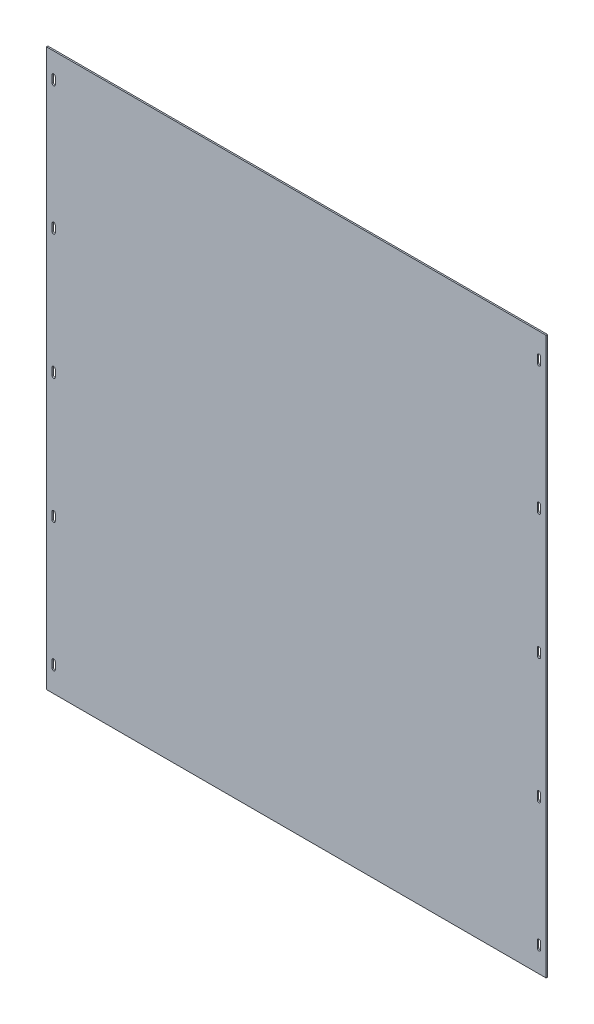
SolidWorks part; units mm, degrees
material "Q235A"
ref_plane "前视基准面" through (0, 0, 0) normal (0, 0, 1) x (1, 0, 0)
ref_plane "上视基准面" through (0, 0, 0) normal (0, 1, 0) x (1, 0, 0)
ref_plane "右视基准面" through (0, 0, 0) normal (1, 0, 0) x (0, 0, -1)
sketch "草图1" plane through (0, 0, 0) normal (0, 0, 1) x (1, 0, 0)
  line L1 (-350, 390) -> (350, 390)
  line L2 (-350, 390) -> (-350, -390)
  line L3 (-350, -390) -> (350, -390)
  line L4 (350, 390) -> (350, -390)
  line L5 (0, -390) -> (0, 390) construction
  line L6 (-350, 0) -> (350, 0) construction
  point P0 (0, 0)
  dimension "D1" = 700
  dimension "D2" = 780
extrude "凸台-拉伸1" add sketch "草图1" along normal blind 2
sketch "草图2" plane through (0, 0, 2) normal (0, 0, 1) x (1, 0, 0)
  line L0 (0, 390) -> (0, -390) construction
  line L1 (350, 390) -> (-350, 390) construction
  line L2 (-350, -390) -> (350, -390) construction
  line L3 (-340, 360) -> (-340, 350) construction
  line L4 (-340, -355) -> (340, -355) construction
  line L5 (-340, -355) -> (-340, 355) construction
  line L6 (-340, 355) -> (340, 355) construction
  line L7 (340, -355) -> (340, 355) construction
  line L8 (0, 355) -> (0, -355) construction
  line L9 (-340, 0) -> (340, 0) construction
  line L10 (-337.75, 360) -> (-337.75, 350)
  line L11 (-342.25, 360) -> (-342.25, 350)
  line L12 (340, 360) -> (340, 350) construction
  line L13 (337.75, 360) -> (337.75, 350)
  line L14 (342.25, 360) -> (342.25, 350)
  line L15 (-340, 170) -> (-340, 180) construction
  line L16 (-342.25, 170) -> (-342.25, 180)
  line L17 (-337.75, 170) -> (-337.75, 180)
  line L18 (-340, -5) -> (-340, 5) construction
  line L19 (-342.25, -5) -> (-342.25, 5)
  line L20 (-337.75, -5) -> (-337.75, 5)
  line L21 (340, 170) -> (340, 180) construction
  line L22 (342.25, 170) -> (342.25, 180)
  line L23 (337.75, 170) -> (337.75, 180)
  line L24 (340, -5) -> (340, 5) construction
  line L25 (342.25, -5) -> (342.25, 5)
  line L26 (337.75, -5) -> (337.75, 5)
  line L27 (-340, 540) -> (-340, 530) construction
  line L28 (-342.25, 540) -> (-342.25, 530)
  line L29 (-337.75, 540) -> (-337.75, 530)
  line L30 (340, 540) -> (340, 530) construction
  line L31 (342.25, 540) -> (342.25, 530)
  line L32 (337.75, 540) -> (337.75, 530)
  line L33 (-340, -355) -> (340, -355) construction
  line L34 (340, -170) -> (340, -180) construction
  line L35 (342.25, -170) -> (342.25, -180)
  line L36 (337.75, -170) -> (337.75, -180)
  line L37 (-340, -170) -> (-340, -180) construction
  line L38 (-342.25, -170) -> (-342.25, -180)
  line L39 (-337.75, -170) -> (-337.75, -180)
  line L40 (340, -360) -> (340, -350) construction
  line L41 (337.75, -360) -> (337.75, -350)
  line L42 (342.25, -360) -> (342.25, -350)
  line L43 (-340, -360) -> (-340, -350) construction
  line L44 (-337.75, -360) -> (-337.75, -350)
  line L45 (-342.25, -360) -> (-342.25, -350)
  arc A0 (-337.75, 360) -> (-342.25, 360) centre (-340, 360) ccw
  arc A1 (-342.25, 350) -> (-337.75, 350) centre (-340, 350) ccw
  arc A2 (337.75, 360) -> (342.25, 360) centre (340, 360) cw
  arc A3 (342.25, 350) -> (337.75, 350) centre (340, 350) cw
  arc A4 (-342.25, 170) -> (-337.75, 170) centre (-340, 170) ccw
  arc A5 (-337.75, 180) -> (-342.25, 180) centre (-340, 180) ccw
  arc A6 (-342.25, -5) -> (-337.75, -5) centre (-340, -5) ccw
  arc A7 (-337.75, 5) -> (-342.25, 5) centre (-340, 5) ccw
  arc A8 (342.25, 170) -> (337.75, 170) centre (340, 170) cw
  arc A9 (337.75, 180) -> (342.25, 180) centre (340, 180) cw
  arc A10 (342.25, -5) -> (337.75, -5) centre (340, -5) cw
  arc A11 (337.75, 5) -> (342.25, 5) centre (340, 5) cw
  arc A12 (-342.25, 540) -> (-337.75, 540) centre (-340, 540) cw
  arc A13 (-337.75, 530) -> (-342.25, 530) centre (-340, 530) cw
  arc A14 (342.25, 540) -> (337.75, 540) centre (340, 540) ccw
  arc A15 (337.75, 530) -> (342.25, 530) centre (340, 530) ccw
  arc A16 (342.25, -170) -> (337.75, -170) centre (340, -170) ccw
  arc A17 (337.75, -180) -> (342.25, -180) centre (340, -180) ccw
  arc A18 (-342.25, -170) -> (-337.75, -170) centre (-340, -170) cw
  arc A19 (-337.75, -180) -> (-342.25, -180) centre (-340, -180) cw
  arc A20 (337.75, -360) -> (342.25, -360) centre (340, -360) ccw
  arc A21 (342.25, -350) -> (337.75, -350) centre (340, -350) ccw
  arc A22 (-337.75, -360) -> (-342.25, -360) centre (-340, -360) cw
  arc A23 (-342.25, -350) -> (-337.75, -350) centre (-340, -350) cw
  point P6 (0, 0)
  point P12 (-340, 355)
  point P19 (340, 355)
  point P26 (-340, 175)
  point P32 (-340, 0)
  point P40 (340, 175)
  point P47 (340, 0)
  point P54 (-340, 535)
  point P61 (340, 535)
  point P68 (340, -175)
  point P75 (-340, -175)
  point P82 (340, -355)
  point P89 (-340, -355)
  dimension "D1" = 680
  dimension "D2" = 710
  dimension "D3" = 4.5
  dimension "D4" = 10
  dimension "D5" = 10
  dimension "D6" = 10
  dimension "D7" = 4.5
  dimension "D8" = 4.5
  dimension "D9" = 175
extrude "切除-拉伸1" cut sketch "草图2" against normal blind 10
